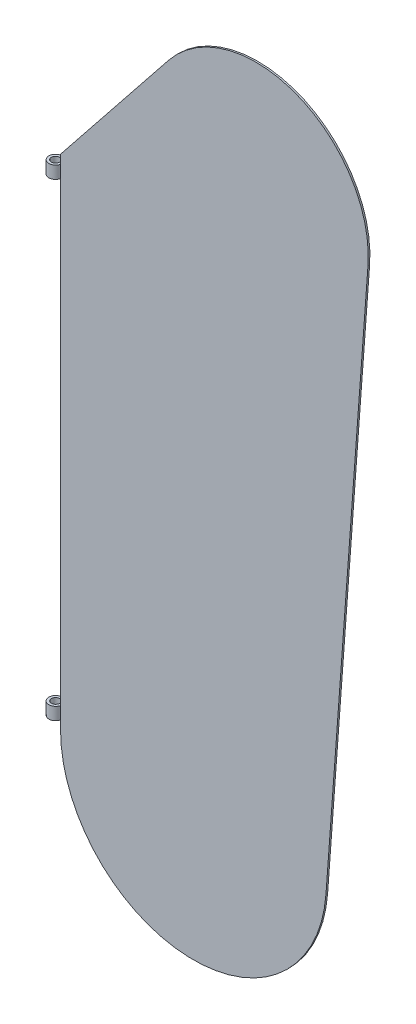
SolidWorks part; units mm, degrees
ref_plane "前视基准面" through (0, 0, 0) normal (0, 0, 1) x (1, 0, 0)
ref_plane "上视基准面" through (0, 0, 0) normal (0, 1, 0) x (1, 0, 0)
ref_plane "右视基准面" through (0, 0, 0) normal (1, 0, 0) x (0, 0, -1)
other "Configuration Table"
sketch "草图1" plane through (0, 0, 0) normal (0, 0, 1) x (1, 0, 0)
  line L0 (134.56, -336.8574) -> (185.1288, 343.6273)
  line L1 (-55.0088, 437.8512) -> (-185, 275)
  line L2 (-185, 275) -> (-185, -325)
  arc A0 (-185, -325) -> (134.56, -336.8574) centre (-25, -325) ccw
  arc A1 (185.1288, 343.6273) -> (-55.0088, 437.8512) centre (50.5, 353.6319) ccw
  dimension "D1" = 135
  dimension "D2" = 160
  dimension "D3" = 600
  dimension "D4" = 4.25
  dimension "D5" = 185
  dimension "D6" = 680.4847
  dimension "D7" = 275
  dimension "D8" = 325
  dimension "D9" = 353.6319
extrude "凸台-拉伸1" add sketch "草图1" along normal blind 2
ref_plane "基准面1" through (0, -325, 0) normal (0, 1, 0) x (1, 0, 0)
ref_plane "基准面2" through (0, -315, 0) normal (0, 1, 0) x (1, 0, 0)
sketch "草图2" plane through (0, -315, 0) normal (0, 1, 0) x (1, 0, 0)
  line L0 (-185, -2) -> (-185, 0) construction
  line L2 (-185, -2) -> (134.56, -2) construction
  circle A0 centre (-193, 0) radius 8
  dimension "D1" = 16
  dimension "D2" = 2
extrude "凸台-拉伸2" add sketch "草图2" along normal blind 15 separate body
ref_plane "基准面3" through (0, 264.3, 0) normal (0, 1, 0) x (1, 0, 0)
sketch "草图3" plane through (0, 264.3, 0) normal (0, 1, 0) x (1, 0, 0)
  circle A0 centre (-193, 0) radius 8
  dimension "D1" = 16
extrude "凸台-拉伸3" add sketch "草图3" against normal blind 15 separate body
sketch "草图5" plane through (0, 264.3, 0) normal (0, 1, 0) x (1, 0, 0)
  circle A0 centre (-193, 0) radius 5
  dimension "D1" = 10
extrude "切除-拉伸1" cut sketch "草图5" against normal through all both and the other way through all
